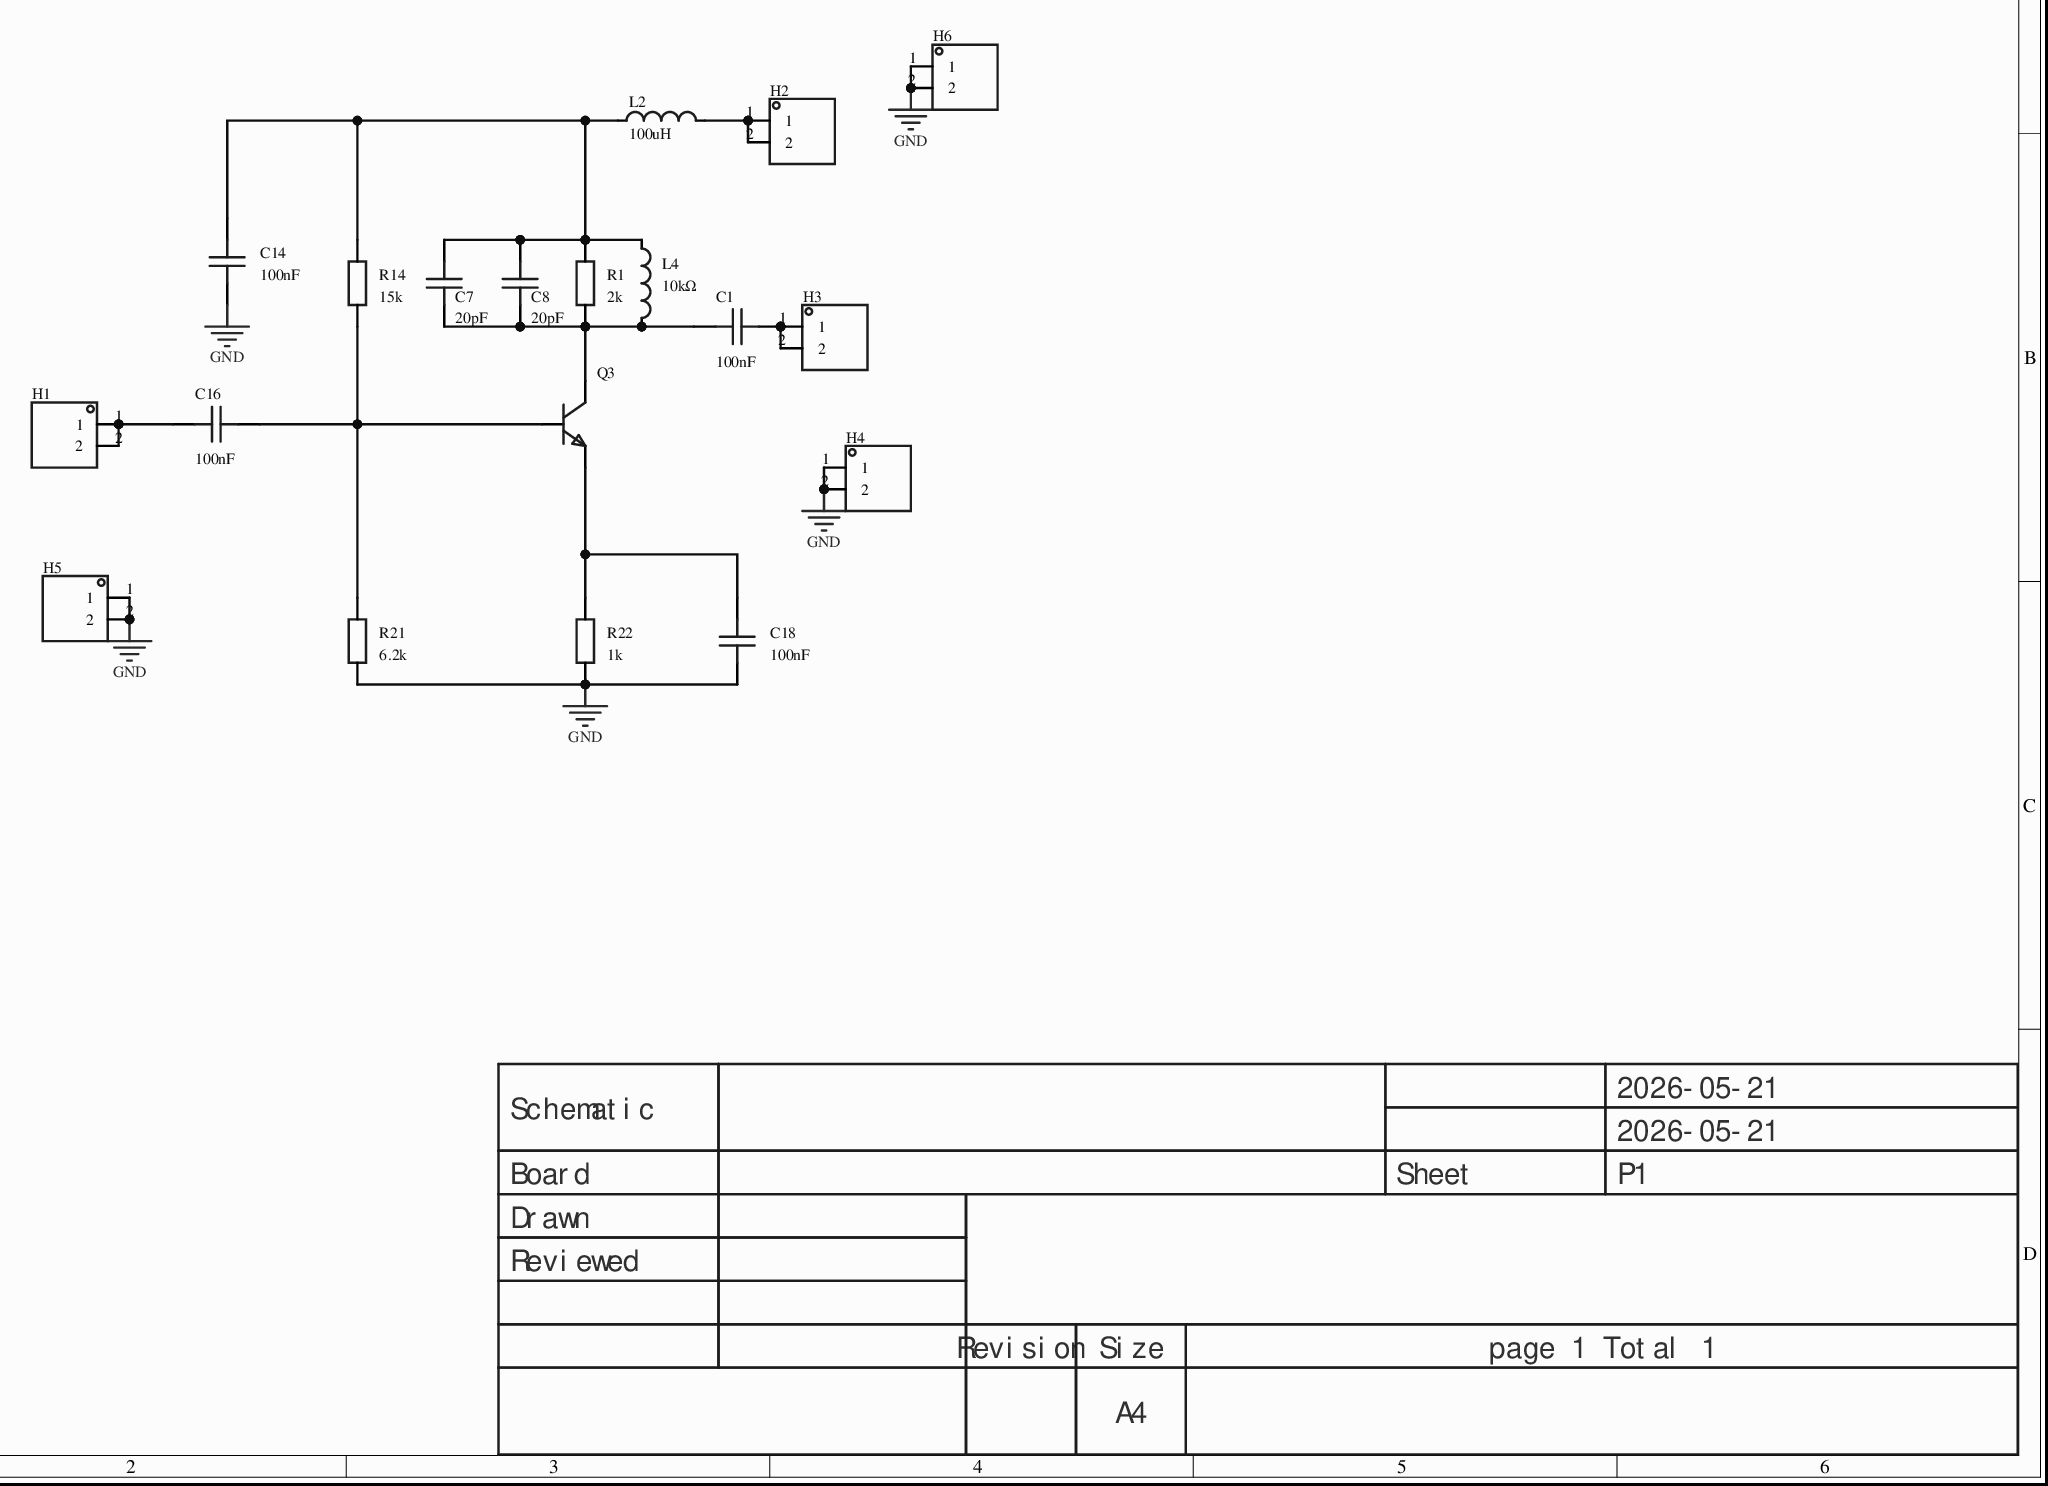
[diagram p0: MISC51307-3.schdoc]
# Altium project MISC51307-2.PrjPcb
1 sheet, 19 parts. Net scope: global (net labels, ports and power ports of the same name join across sheets).
Board file: MISC51307.pcbdoc

## Sheet MISC51307-3.schdoc
size 297 x 209 mm; Version: V1.0; @Project Name: MISC51307; @Update Date: 2026-05-21; @Create Date: 2026-05-21; @Board Name: MISC51307; @Create Time: 23:10:26; @Page Count: 1; @Page No: 1; @Schematic Name: MISC51307; @Update Time: 23:10:26; Size: A4

### Parts
C1  100nF  [C0805]
C7  20pF  [C0805]
C8  20pF  [C0805]
C14  100nF  [C0805]
C16  100nF  [C0805]
C18  100nF  [C0805]
H1  (no value)  [HDR-TH_2P-P2.54-V-M-1]
H2  (no value)  [HDR-TH_2P-P2.54-V-M-1]
H3  (no value)  [HDR-TH_2P-P2.54-V-M-1]
H4  (no value)  [HDR-TH_2P-P2.54-V-M-1]
H5  (no value)  [HDR-TH_2P-P2.54-V-M-1]
H6  (no value)  [HDR-TH_2P-P2.54-V-M-1]
L2  100uH  [IND-SMD_L5.8-W5.2]
L4  10kΩ  [Res_1/4W]
Q3  (no value)  [S8050_TO_92]
R1  2k  [R0805]
R14  15k  [R0805]
R21  6.2k  [R0805]
R22  1k  [R0805]

### Nets
GND: C14.1 C18.2 H4.1 H4.2 H5.1 H5.2 H6.1 H6.2 R21.1 R22.1
NetC1_1: C1.1 C7.1 C8.1 L4.1 Q3.3(C) R1.1
NetC1_2: C1.2 H3.1 H3.2
NetC7_2: C7.2 C8.2 C14.2 L2.1 L4.2 R1.2 R14.2
NetC16_1: C16.1 Q3.2(B) R14.1 R21.2
NetC16_2: C16.2 H1.1 H1.2
NetC18_1: C18.1 Q3.1(E) R22.2
NetH2_1: H2.1 H2.2 L2.2

### Notes on the sheet
- 2026-05-21
- Schematic
- Board
- Sheet
- P1
- Drawn
- Reviewed
- Revision
- Size
- A4
- page 1 Total 1

### Library data of the parts
C1 C7 C8 C14 C16 C18 = CAP_0603: Symbol: Capacitance; ConvertToPcb: yes; ModelId: ac125912035d415993ca9572d50418b10819f05c4eef4c71ace90d822a990e87; ModelName: C0603_L1.6-W0.8-H0.8; ModelTransform: 62.992,31.496,0,0,0,0,0,0,0; Device: CAP_0603; AddInBom: yes; Supplier Footprint: 0603; FootprintName: C0805
  C1 C14 C16 C18: Value: 100nF
  C7 C8: Value: 20pF
H1-H6 = HDR-M_2.54_1x2P: Symbol: 210S-1*2P L=11.6MMGold-plated black; ConvertToPcb: yes; ModelId: 79b2e9f2d70a4d68a1b7098f27c6d4c50819f05c4eef4c71ace90d822a990e87; ModelName: HDR-M-2.54_1x2; ModelTransform: 200,100,0,0,0,0,0,0,-118.11; Device: HDR-M_2.54_1x2P; AddInBom: yes; SupplierPart: C124375; Supplier Footprint: 插件; FootprintName: HDR-TH_2P-P2.54-V-M-1
L2 = INDUCTOR_CD54: SMD wire-wound inductor; Manufacturer: DMBJ(振宝佳); AddInBom: yes; ModelId: a8dd117e79f74e3dbd87b6fac5eb2c6776145ff29cae4c63908fb42ebdf03575; ModelName: IND-SMD_L5.8-W5.2-H4.5; ModelTransform: 209.049,228.346,0,90,0,0,0.994,0,0; Symbol: INDUCTOR_CD54; Device: INDUCTOR_CD54; Value: 100uH; Datasheet: https://atta.szlcsc.com/upload/public/pdf/source/20210416/C2826610_BD9EF4281FEC8102FBF66339CC69A197.pdf; ConvertToPcb: yes; FootprintName: IND-SMD_L5.8-W5.2
L4 = Res_AXIAL-1/4W: Symbol: Resistor_1; AddInBom: yes; ModelId: 463263665006444ab7a47bd11b0cf9560819f05c4eef4c71ace90d822a990e87; ModelName: RES-TH_BD2.4-L6.3-P10.30-D0.6; ModelTransform: 427.165,94.32816,0,0,0,0,0,0,-196.85; Device: Res_AXIAL-1/4W; Supplier Footprint: 轴向引线; ConvertToPcb: yes; FootprintName: Res_1/4W; Value: 10kΩ
Q3 = S8050_TO_NPN: ConvertToPcb: yes; ModelId: aafe8e06f2154e7c93506efd0d6632dd0819f05c4eef4c71ace90d822a990e87; ModelName: TO-92-3_L4.9-W3.7-P1.27-L; ModelTransform: 180.78,141.44,417.3,0,0,0,0,0,-200; Symbol: S8050_TO_NPN; Device: S8050_TO_NPN; AddInBom: yes; Supplier Footprint: TO-92; FootprintName: S8050_TO_92
R1 R14 R21 R22 = Res_0603: Symbol: Resistor; ConvertToPcb: yes; ModelId: fc143cca1e79419f9cd78b61e9279f080819f05c4eef4c71ace90d822a990e87; ModelName: R0603; ModelTransform: 31.8897,63.7794,0,90,0,0,0,0,0; Device: Res_0603; AddInBom: yes; Supplier Footprint: 0603; FootprintName: R0805
  R1: Value: 2k
  R14: Value: 15k
  R21: Value: 6.2k
  R22: Value: 1k